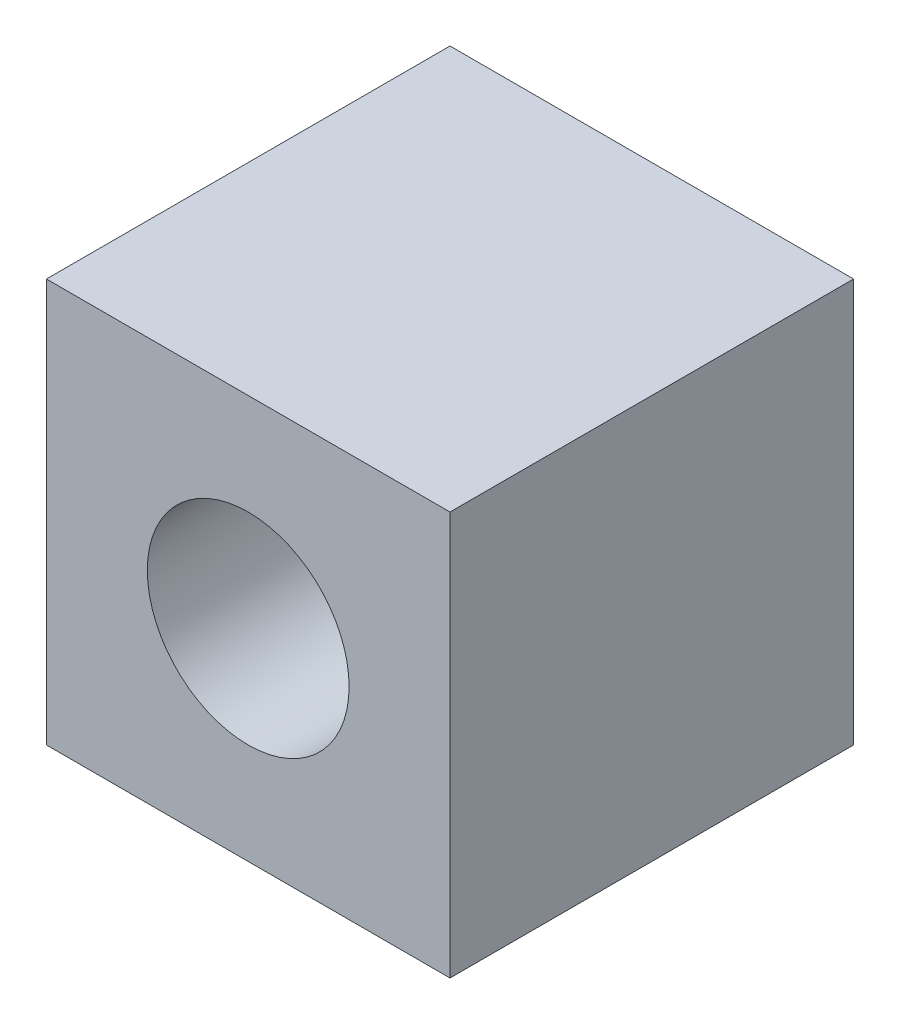
from build123d import *

# Parameters (mm, degrees)
SKETCH1_W          = 20
SKETCH1_H          = 20
BASE_EXTRUDE_DEPTH = 20
SKETCH2_R          = 5
CUT_EXTRUDE1_DEPTH = 25.494897428


with BuildPart() as part:
    # Sketch1 → Base-Extrude (new body)
    with BuildSketch(Plane.XY):
        Rectangle(SKETCH1_W, SKETCH1_H)
    extrude(amount=BASE_EXTRUDE_DEPTH)

    # Sketch2 → Cut-Extrude1 (cut, through all)
    with BuildSketch(Plane.XY.offset(20)):
        Circle(SKETCH2_R)
    extrude(amount=-CUT_EXTRUDE1_DEPTH, mode=Mode.SUBTRACT)


solid = part.part
